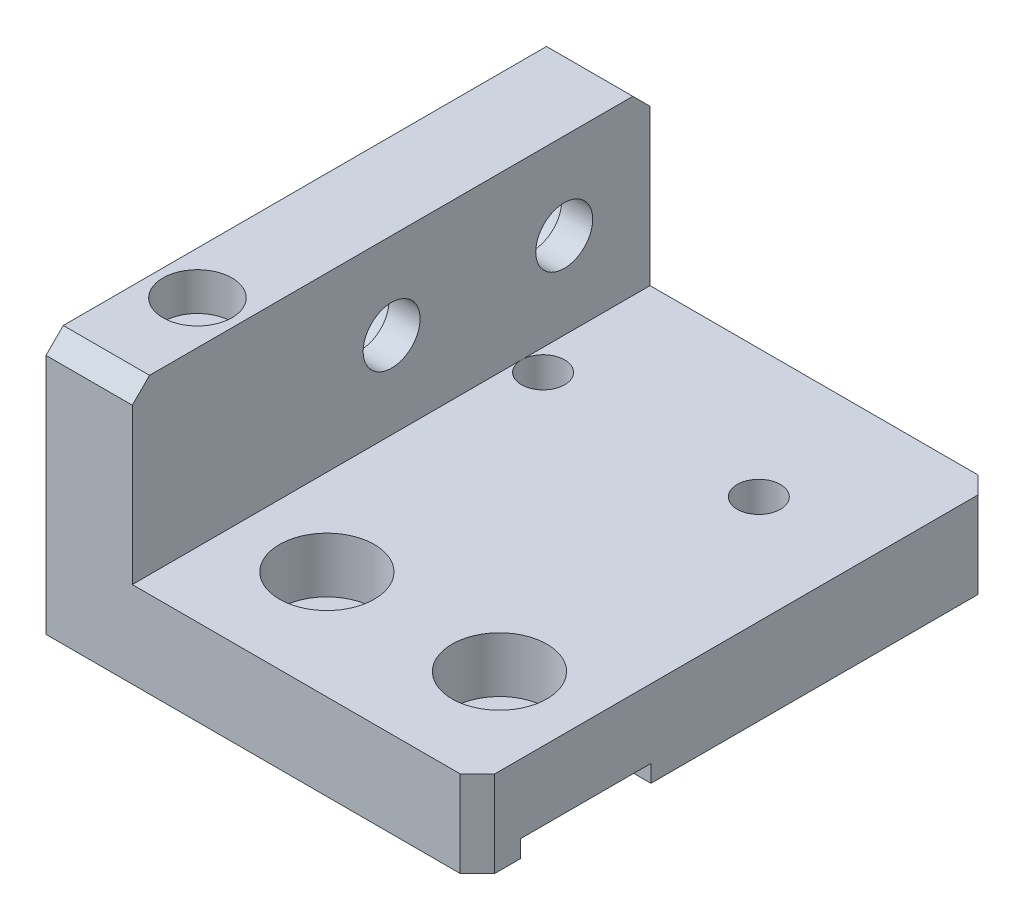
SolidWorks part; units mm, degrees
material "6061-T6"
ref_plane "前视基准面" through (0, 0, 0) normal (0, 0, 1) x (1, 0, 0)
ref_plane "上视基准面" through (0, 0, 0) normal (0, 1, 0) x (1, 0, 0)
ref_plane "右视基准面" through (0, 0, 0) normal (1, 0, 0) x (0, 0, -1)
sketch "草图2" plane through (0, 0, 0) normal (0, 0, 1) x (1, 0, 0)
  line L0 (50, 0) -> (0, 0)
  line L1 (0, 0) -> (0, 30)
  line L2 (50, 10) -> (10, 10)
  line L3 (10, 10) -> (10, 30)
  line L4 (10, 30) -> (0, 30)
  line L5 (50, 10) -> (50, 0)
  dimension "D1" = 50
  dimension "D2" = 30
  dimension "D3" = 10
extrude "凸台-拉伸1" add sketch "草图2" along normal blind 60
sketch "草图3" plane through (0, 0, 0) normal (0, -1, 0) x (1, 0, 0)
  line L0 (0, 60) -> (0, 0) construction
  line L1 (0, 55) -> (50, 55)
  line L2 (0, 55) -> (0, 39.9)
  line L3 (0, 39.9) -> (50, 39.9)
  line L4 (50, 55) -> (50, 39.9)
  line L5 (50, 60) -> (50, 0) construction
  line L6 (0, 60) -> (50, 60) construction
  dimension "D1" = 15.1
  dimension "D2" = 5
extrude "切除-拉伸1" cut sketch "草图3" against normal blind 2
hole_wizard "M4 六角凹头螺钉的柱形沉头孔1" positions "草图6" profile "草图8" counterbore size "M4" standard "ISO" end condition through all
sketch "草图6" plane through (-8.9755, 30, 41.4767) normal (0, 1, 0) x (1, 0, 0)
  line L9 (33.9755, 1.5767) -> (33.9755, -13.5233) construction
  line L10 (8.9755, 1.5767) -> (58.9755, 1.5767) construction
  line L11 (58.9755, -13.5233) -> (8.9755, -13.5233) construction
  line L13 (13.9755, -5.9733) -> (33.9755, -5.9733) construction
  line L15 (13.9755, -5.9733) -> (13.9755, -18.5233) construction
  line L16 (18.9755, -18.5233) -> (8.9755, -18.5233) construction
  point P0 (13.9755, -5.9733)
sketch "草图8" plane through (5, 30, 47.45) normal (1, 0, 0) x (0, 0, 1)
  line L0 (0, 0) -> (0, 30)
  line L1 (0, 30) -> (2.25, 30)
  line L3 (2.25, 30) -> (2.25, 4.4)
  line L4 (2.25, 4.4) -> (4, 4.4)
  line L5 (4, 4.4) -> (4, 0)
  line L7 (4, 0) -> (0, 0)
  line L11 (0, -6.35) -> (0, 107.95) construction
  dimension "通孔孔直径" = 4.5
  dimension "通孔孔深度" = 30
  dimension "柱形沉头孔直径" = 8
  dimension "柱形沉头孔深度" = 4.4
hole_wizard "M6 六角凹头螺钉的柱形沉头孔1" positions "草图10" profile "草图12" counterbore size "M6" standard "ISO" end condition through all
sketch "草图10" plane through (0, 10, 0) normal (0, 1, 0) x (1, 0, 0)
  line L0 (40, -47.45) -> (20, -47.45) construction
  line L1 (20, -47.45) -> (5, -47.45) construction
  line L3 (30, -47.45) -> (30, 0) construction
  line L5 (50, 0) -> (10, 0) construction
  point P0 (20, -47.45)
  point P2 (40, -47.45)
  dimension "D1" = 20
sketch "草图12" plane through (20, 10, 47.45) normal (1, 0, 0) x (0, 0, 1)
  line L0 (0, 0) -> (0, 10)
  line L1 (0, 10) -> (3.3, 10)
  line L3 (3.3, 10) -> (3.3, 6.4)
  line L4 (3.3, 6.4) -> (5.5, 6.4)
  line L5 (5.5, 6.4) -> (5.5, 0)
  line L7 (5.5, 0) -> (0, 0)
  line L11 (0, -6.35) -> (0, 107.95) construction
  dimension "通孔孔直径" = 6.6
  dimension "通孔孔深度" = 10
  dimension "柱形沉头孔直径" = 11
  dimension "柱形沉头孔深度" = 6.4
hole_wizard "M6 六角凹头螺钉的柱形沉头孔2" positions "草图13" profile "草图14" counterbore size "M6" standard "ISO" end condition through all
sketch "草图13" plane through (0, 0, 0) normal (-1, 0, 0) x (0, 0, 1)
  line L4 (9.95, 20) -> (29.95, 20) construction
  line L6 (19.95, 20) -> (19.95, 0) construction
  line L8 (60, 30) -> (0, 30) construction
  line L9 (39.9, 0) -> (0, 0) construction
  point P0 (9.95, 20)
  point P2 (29.95, 20)
  dimension "D1" = 20
  dimension "D2" = 10
sketch "草图14" plane through (0, 20, 9.95) normal (0, 1, 0) x (0, 0, 1)
  line L0 (0, 0) -> (0, 50)
  line L1 (0, 50) -> (3.3, 50)
  line L3 (3.3, 50) -> (3.3, 6.4)
  line L4 (3.3, 6.4) -> (5.5, 6.4)
  line L5 (5.5, 6.4) -> (5.5, 0)
  line L7 (5.5, 0) -> (0, 0)
  line L11 (0, -6.35) -> (0, 107.95) construction
  dimension "通孔孔直径" = 6.6
  dimension "通孔孔深度" = 50
  dimension "柱形沉头孔直径" = 11
  dimension "柱形沉头孔深度" = 6.4
chamfer "倒角1" distance 2 angle 45 4 edges at (50, 5, 60) (50, 5, 0) (5, 30, 0) (5, 30, 60)
hole_wizard "M6 螺纹孔1" positions "草图15" profile "草图16" tap size "M6" standard "ISO"
sketch "草图15" plane through (0, 0, 0) normal (0, -1, 0) x (-1, 0, 0)
  line L0 (-37.5, -14.9) -> (-12.5, -14.9) construction
  line L2 (0, 0) -> (-48, 0) construction
  line L4 (-25, -14.9) -> (-25, -22.8599) construction
  line L6 (-50, -39.9) -> (-50, -2) construction
  point P0 (-12.5, -14.9)
  point P2 (-37.5, -14.9)
  dimension "D1" = 14.9
  dimension "D2" = 25
  dimension "D3" = 25
sketch "草图16" plane through (12.5, 0, 14.9) normal (1, 0, 0) x (0, 0, -1)
  line L0 (0, 0) -> (0, 18.5022)
  line L1 (0, 18.5022) -> (2.5, 17)
  line L2 (2.5, 17) -> (2.5, 0)
  line L5 (2.5, 0) -> (0, 0)
  line L10 (0, 18.5022) -> (-2.5, 17) construction
  line L11 (0, -6.35) -> (0, 107.95) construction
  dimension "螺纹孔钻头直径" = 5
  dimension "螺纹孔钻头深度" = 17
  dimension "导头角度" = 118
cosmetic thread "孔螺蚊线1" parameters "D1"=10, "D2"=6
cosmetic thread "孔螺蚊线2" parameters "D1"=12, "D2"=6
